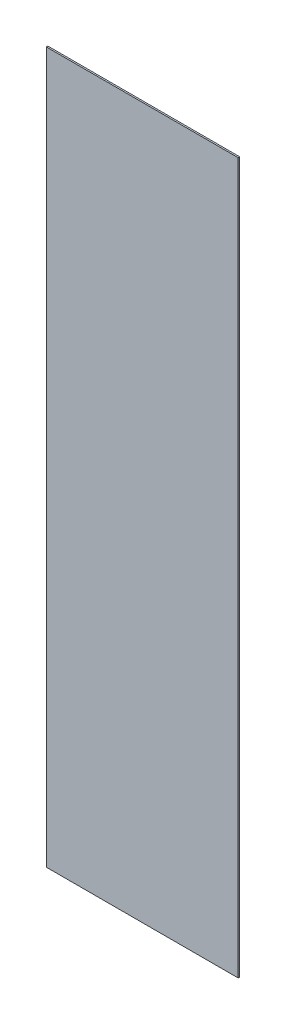
SolidWorks part; units mm, degrees
material "PMMA(有机玻璃)"
ref_plane "前视" through (0, 0, 0) normal (0, 0, 1) x (1, 0, 0)
ref_plane "上视" through (0, 0, 0) normal (0, 1, 0) x (1, 0, 0)
ref_plane "右视" through (0, 0, 0) normal (1, 0, 0) x (0, 0, -1)
sketch "草图1" plane through (0, 0, 0) normal (0, 0, 1) x (1, 0, 0)
  line L1 (-312, 1155) -> (312, 1155)
  line L2 (-312, 1155) -> (-312, -1155)
  line L3 (-312, -1155) -> (312, -1155)
  line L4 (312, 1155) -> (312, -1155)
  line L5 (-312, 1155) -> (312, -1155) construction
  line L6 (-312, -1155) -> (312, 1155) construction
  point P0 (0, 0)
  dimension "D1" = 2310
  dimension "D2" = 624
extrude "凸台-拉伸1" add sketch "草图1" along normal blind 5
hole_wizard "M5 间隙孔1" positions "草图3" profile "草图2" hole size "M5" standard "GB"
sketch "草图3" plane through (0, 0, 5) normal (0, 0, 1) x (1, 0, 0)
  line L0 (-427.5, 273) -> (-427.5, -273) construction
  line L1 (-427.5, -273) -> (427.5, -273) construction
  line L2 (0, 273) -> (0, -273) construction
  line L3 (427.5, 273) -> (-427.5, 273) construction
  line L5 (-427.5, 0) -> (427.5, 0) construction
  line L6 (427.5, -273) -> (427.5, 273) construction
  point P0 (-375, -261)
  point P46 (415.5, 250)
  point P48 (-415.5, 250)
  point P58 (-125, -261)
  point P59 (125, -261)
  point P61 (-125, 261)
  point P62 (125, 261)
  point P64 (-375, 261)
  point P88 (375, -261)
  point P89 (375, 261)
  point P108 (415.5, 0)
  point P109 (-415.5, 0)
  point P110 (415.5, -250)
  point P111 (-415.5, -250)
  dimension "D1" = 12
  dimension "D2" = 12
  dimension "D5" = 3
  dimension "D3" = 12
  dimension "D6" = 4
  dimension "D4" = 2
sketch "草图2" plane through (-375, -261, 5) normal (1, 0, 0) x (0, -1, 0)
  line L0 (0, 0) -> (0, 5)
  line L1 (0, 5) -> (2.75, 5)
  line L2 (2.75, 5) -> (2.75, 0)
  line L5 (2.75, 0) -> (0, 0)
  line L11 (0, -6.35) -> (0, 107.95) construction
  dimension "通孔孔直径" = 5.5
  dimension "通孔孔深度" = 5
